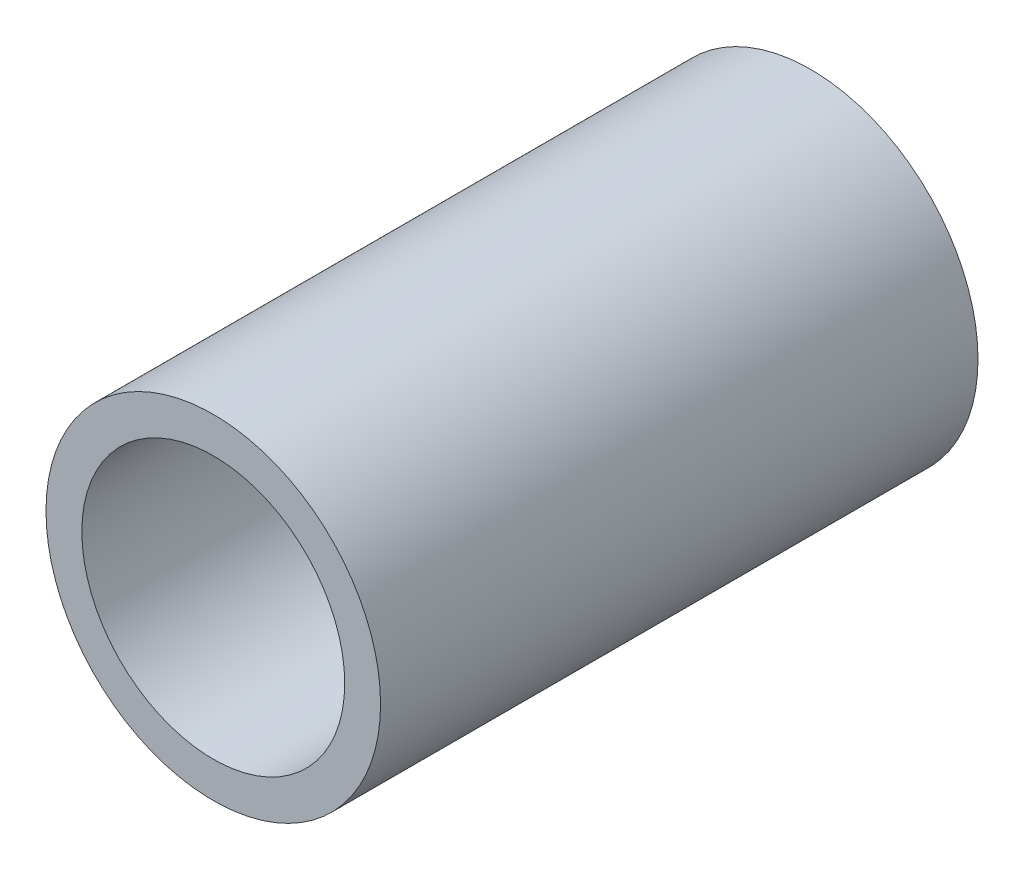
SolidWorks part; units mm, degrees
ref_plane "前视基准面" through (0, 0, 0) normal (0, 0, 1) x (1, 0, 0)
ref_plane "上视基准面" through (0, 0, 0) normal (0, 1, 0) x (1, 0, 0)
ref_plane "右视基准面" through (0, 0, 0) normal (1, 0, 0) x (0, 0, -1)
other "Configuration Table"
sketch "草图1" plane through (0, 0, 0) normal (0, 0, 1) x (1, 0, 0)
  circle A0 centre (0, 0) radius 28
  circle A1 centre (0, 0) radius 22
  point P0 (0, 0)
  dimension "D1" = 44
  dimension "D2" = 56
extrude "凸台-拉伸1" add sketch "草图1" against normal mid plane 100
